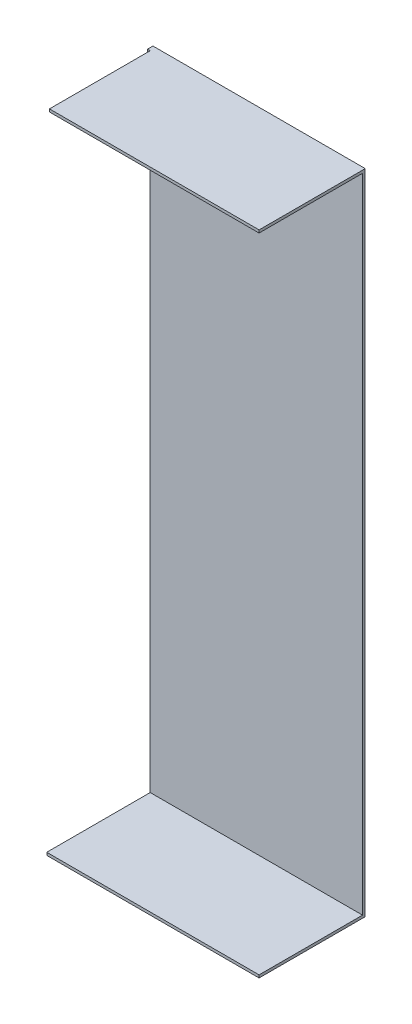
SolidWorks part; units mm, degrees
ref_plane "Front Plane" through (0, 0, 0) normal (0, 0, 1) x (1, 0, 0)
ref_plane "Top Plane" through (0, 0, 0) normal (0, 1, 0) x (1, 0, 0)
ref_plane "Right Plane" through (0, 0, 0) normal (1, 0, 0) x (0, 0, -1)
sketch "Sketch1" plane through (0, 0, 0) normal (0, 0, 1) x (1, 0, 0)
  line L1 (-38.5, 119) -> (38.5, 119)
  line L2 (-38.5, 119) -> (-38.5, -119)
  line L3 (-38.5, -119) -> (38.5, -119)
  line L4 (38.5, 119) -> (38.5, -119)
  line L5 (-38.5, 119) -> (38.5, -119) construction
  line L6 (-38.5, -119) -> (38.5, 119) construction
  point P0 (0, 0)
  dimension "D1" = 77
  dimension "D2" = 238
extrude "Boss-Extrude1" add sketch "Sketch1" along normal blind 1
sketch "Sketch2" plane through (0, 0, 1) normal (0, 0, 1) x (1, 0, 0)
  line L0 (38.5, -119) -> (38.5, 119) construction
  line L1 (-38.5, 119) -> (38.5, 119)
  line L2 (-38.5, 119) -> (-38.5, 118)
  line L3 (-38.5, 118) -> (38.5, 118)
  line L4 (38.5, 119) -> (38.5, 118)
  line L5 (0, 0) -> (88.4377, 0) construction
  line L6 (38.5, -119) -> (38.5, -118)
  line L7 (-38.5, -118) -> (38.5, -118)
  line L8 (-38.5, -119) -> (-38.5, -118)
  line L9 (-38.5, -119) -> (38.5, -119)
  dimension "D1" = 1
extrude "Boss-Extrude2" add sketch "Sketch2" along normal blind 38
sketch "Sketch3" plane through (-38.5, 0, 0) normal (-1, 0, 0) x (0, 0, 1)
  line L0 (2, 119) -> (0, 119)
  line L1 (0, 119) -> (0, -119) construction
  line L2 (39, 119) -> (0, 119) construction
  line L3 (0, 119) -> (0, -119)
  line L4 (0, -119) -> (39, -119)
  line L5 (39, -119) -> (39, -118)
  line L6 (39, -118) -> (1, -118)
  line L7 (1, -118) -> (1, 118)
  line L8 (1, 118) -> (2, 118)
  line L9 (2, 119) -> (2, 99) construction
  line L10 (39, 118) -> (1, 118) construction
  line L11 (2, 118) -> (2, 119)
extrude "Boss-Extrude3" add sketch "Sketch3" along normal blind 1
